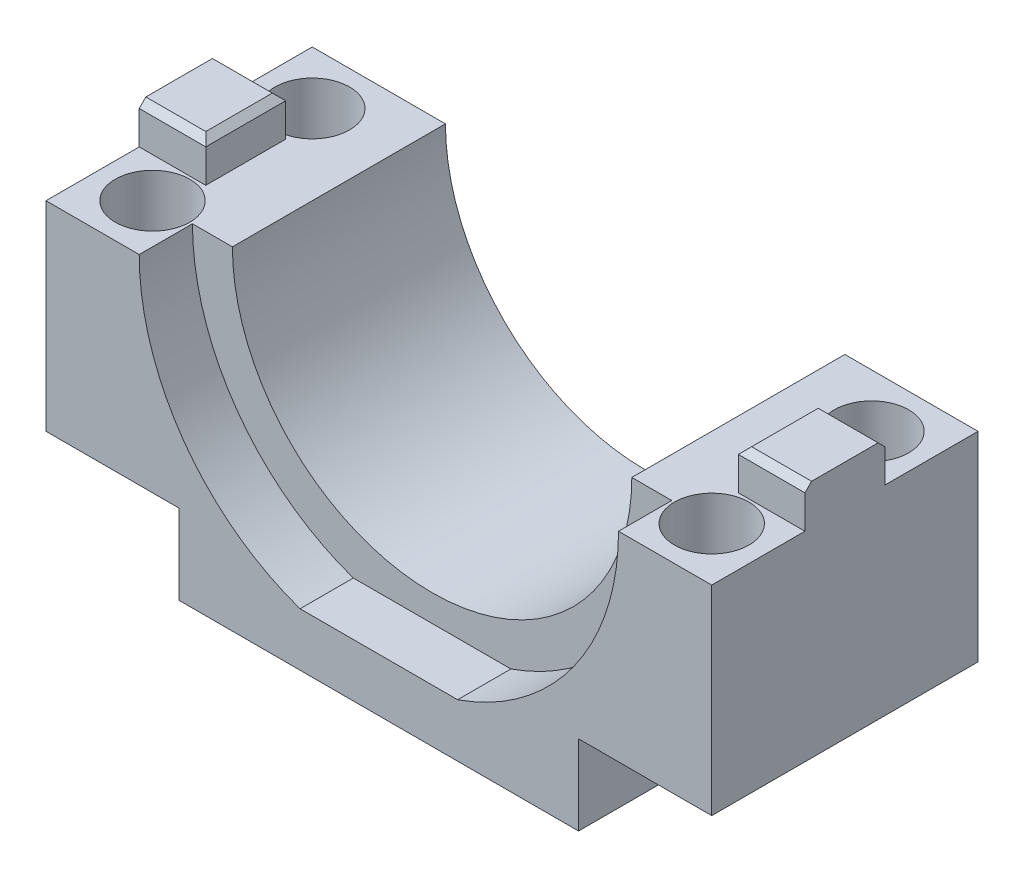
SolidWorks part; units mm, degrees
ref_plane "Front Plane" through (0, 0, 0) normal (0, 0, 1) x (1, 0, 0)
ref_plane "Top Plane" through (0, 0, 0) normal (0, 1, 0) x (1, 0, 0)
ref_plane "Right Plane" through (0, 0, 0) normal (1, 0, 0) x (0, 0, -1)
sketch "Sketch1" plane through (0, 0, 0) normal (0, 0, 1) x (1, 0, 0)
  line L1 (25, 10.5) -> (-25, 10.5)
  line L2 (25, 10.5) -> (25, -10.5)
  line L3 (25, -10.5) -> (-25, -10.5)
  line L4 (-25, 10.5) -> (-25, -10.5)
  line L5 (25, 10.5) -> (-25, -10.5) construction
  line L6 (25, -10.5) -> (-25, 10.5) construction
  point P0 (0, 0)
  dimension "D1" = 21
  dimension "D2" = 50
extrude "Boss-Extrude1" add sketch "Sketch1" along normal blind 20 contours L2 L1 L4 L3
sketch "Sketch2" plane through (0, 0, 20) normal (0, 0, 1) x (1, 0, 0)
  line L0 (25, 10.5) -> (-25, 10.5) construction
  circle A0 centre (0, 10.5) radius 15
  dimension "D1" = 30
extrude "Cut-Extrude1" cut sketch "Sketch2" against normal blind 20
sketch "Sketch3" plane through (0, 0, 20) normal (0, 0, 1) x (1, 0, 0)
  line L0 (0, 0) -> (0, -13.4465) construction
  line L1 (-15, -4.5) -> (-25, -4.5)
  line L2 (-15, -4.5) -> (-15, -10.5)
  line L3 (-15, -10.5) -> (-25, -10.5)
  line L4 (-25, -4.5) -> (-25, -10.5)
  line L5 (-15, -4.5) -> (-25, -10.5) construction
  line L6 (-15, -10.5) -> (-25, -4.5) construction
  line L7 (15, -10.5) -> (25, -4.5) construction
  line L8 (15, -4.5) -> (25, -10.5) construction
  line L9 (25, -4.5) -> (25, -10.5)
  line L10 (15, -10.5) -> (25, -10.5)
  line L11 (15, -4.5) -> (15, -10.5)
  line L12 (15, -4.5) -> (25, -4.5)
  point P0 (-20, -7.5)
  point P13 (20, -7.5)
  dimension "D1" = 6
  dimension "D2" = 10
extrude "Cut-Extrude2" cut sketch "Sketch3" against normal blind 20
sketch "Sketch4" plane through (0, -4.5, 0) normal (0, -1, 0) x (1, 0, 0)
  line L0 (-15, 20) -> (-25, 20) construction
  line L2 (-25, 0) -> (-25, 20) construction
  line L3 (-15, 0) -> (-25, 0) construction
  circle A0 centre (-21, 16) radius 2.8
  circle A1 centre (-21, 4) radius 2.8
  circle A2 centre (21, 16) radius 2.8
  circle A3 centre (21, 4) radius 2.8
  dimension "D5" = 5.6
  dimension "D1" = 4
  dimension "D2" = 42
  dimension "D3" = 4
  dimension "D4" = 4
extrude "Cut-Extrude3" cut sketch "Sketch4" against normal blind 20
sketch "Sketch5" plane through (0, 10.5, 0) normal (0, 1, 0) x (1, 0, 0)
  line L0 (-25, -20) -> (-25, 0) construction
  line L1 (-20, -13) -> (-25, -13)
  line L2 (-20, -13) -> (-20, -7)
  line L3 (-20, -7) -> (-25, -7)
  line L4 (-25, -13) -> (-25, -7)
  line L5 (-20, -13) -> (-25, -7) construction
  line L6 (-20, -7) -> (-25, -13) construction
  line L7 (25, -20) -> (25, 0) construction
  line L8 (0, 0) -> (0, -4.1831) construction
  line L9 (20, -7) -> (25, -13) construction
  line L10 (20, -13) -> (25, -7) construction
  line L11 (25, -13) -> (25, -7)
  line L12 (20, -7) -> (25, -7)
  line L13 (20, -13) -> (20, -7)
  line L14 (20, -13) -> (25, -13)
  point P0 (-22.5, -10)
  point P10 (25, -10)
  point P17 (22.5, -10)
  dimension "D1" = 5
  dimension "D2" = 6
extrude "Boss-Extrude2" add sketch "Sketch5" along normal blind 3
chamfer "Chamfer2" distance 0.5 angle 45 6 edges at (-22.5, 13.5, 7) (-20, 13.5, 10) (-22.5, 13.5, 13) (22.5, 13.5, 13) (20, 13.5, 10) (22.5, 13.5, 7)
sketch "Sketch6" plane through (0, 0, 20) normal (0, 0, 1) x (1, 0, 0)
  line L0 (-5.9161, -6.5) -> (5.9161, -6.5)
  arc A0 (5.9161, -6.5) -> (-5.9161, -6.5) centre (0, 10.5) ccw
  dimension "D1" = 36
  dimension "D2" = 17
extrude "Cut-Extrude4" cut sketch "Sketch6" against normal blind 4
